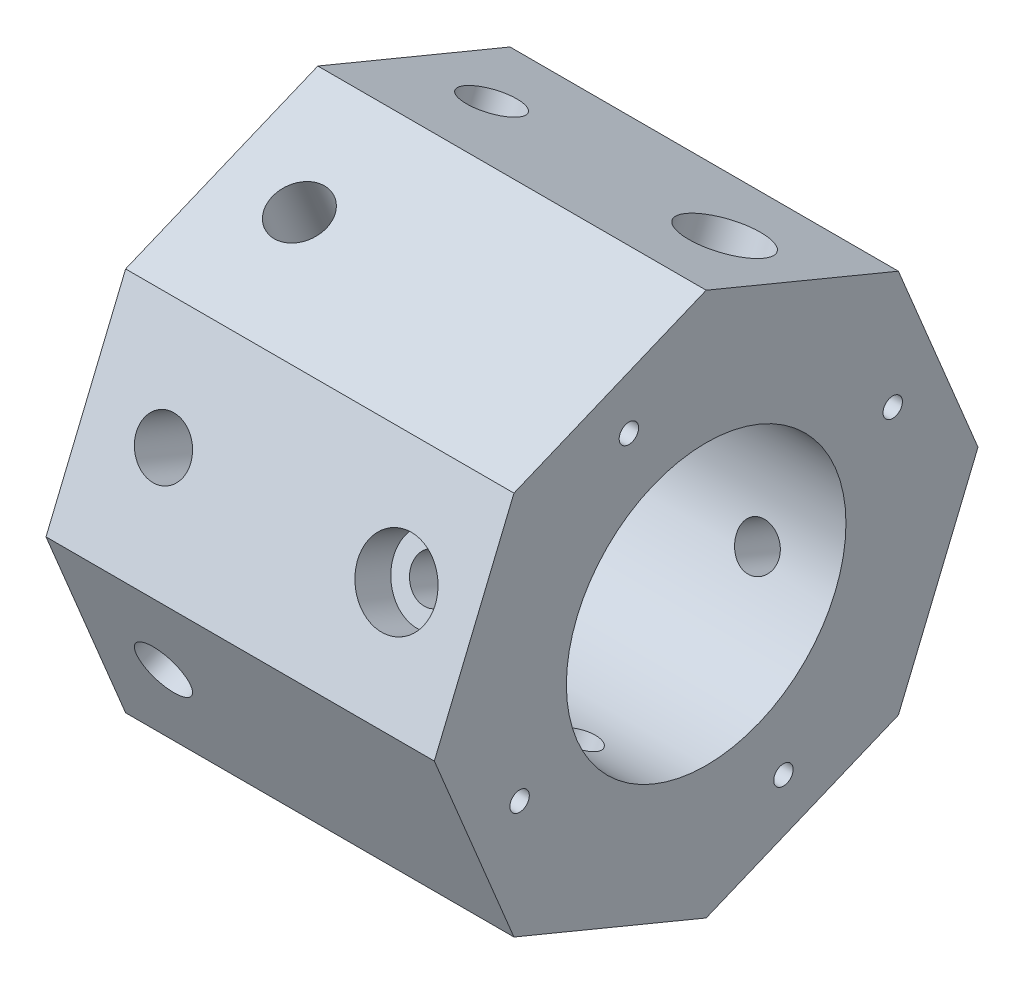
from build123d import *

# Parameters (mm, degrees)
SKETCH_1_R               = 18
EXTRUDE_1_DEPTH          = 25
SKETCH_2_R               = 5
CUT_EXTRUDE_1_DEPTH      = 5
SKETCH_4_R               = 2.75
CUT_EXTRUDE_2_DEPTH      = 23
PATTERN_CIRCULAR_1_COUNT = 8
PATTERN_CIRCULAR_2_COUNT = 4
PATTERN_CIRCULAR_3_COUNT = 4


with BuildPart() as part:
    # 草图1 → 凸台-拉伸1 (new, symmetric)
    with BuildSketch(Plane(origin=(0, 0, 0), x_dir=(0, 0, -1), z_dir=(1, 0, 0))):
        Polygon((24.748737342, 24.748737342), (0, 35), (-24.748737342, 24.748737342), (-35, 0), (-24.748737342, -24.748737342), (0, -35), (24.748737342, -24.748737342), (35, 0), align=None)
        Circle(SKETCH_1_R, mode=Mode.SUBTRACT)
    extrude(amount=EXTRUDE_1_DEPTH, both=True)

    # 草图2 → 切除-拉伸1 (cut)
    with BuildSketch(Plane(origin=(0, -29.874368671, 12.374368671), x_dir=(1, 0, 0), z_dir=(0, 0.9238795325112868, -0.3826834323650897))):
        with Locations(Location((15, 0, 0), (0, 0, 270))):
            Circle(SKETCH_2_R)
    cut_extrude_1 = extrude(amount=CUT_EXTRUDE_1_DEPTH, mode=Mode.SUBTRACT)

    # 草图4 → 切除-拉伸2 (cut)
    with BuildSketch(Plane(origin=(0, -25.254971008, 10.460951509), x_dir=(1, 0, 0), z_dir=(0, -0.9238795325112867, 0.38268343236508956))):
        with Locations(Location((15, 0, 0), (0, 0, 270))):
            Circle(SKETCH_4_R)
    cut_extrude_2 = extrude(amount=-CUT_EXTRUDE_2_DEPTH, mode=Mode.SUBTRACT)

    # 草图6 → M8x1.0 螺纹孔1 (revolve, cut)
    with BuildSketch(Plane(origin=(-15, -12.374368671, 29.874368671), x_dir=(0, -0.9238795325112867, -0.38268343236508995), z_dir=(1, 0, 0))):
        Polygon((0, 0), (0, 17.103012167), (3.5, 15), (3.5, 0), align=None)
    m8x1_0_1 = revolve(axis=Axis((-15, -14.804408466, 35.741003702), (0, 0.38268343236508995, -0.9238795325112867)), mode=Mode.SUBTRACT)

    # 阵列(圆周)1: M8x1.0 螺纹孔1 ×8 about axis
    pattern_circular_1_axis = Axis((25, 0, 0), (-1, 0, 0))
    for i in range(1, PATTERN_CIRCULAR_1_COUNT):
        add(m8x1_0_1.rotate(pattern_circular_1_axis, i * 360 / PATTERN_CIRCULAR_1_COUNT), mode=Mode.SUBTRACT)

    # 阵列(圆周)2: 切除-拉伸1, 切除-拉伸2 ×4 about axis
    pattern_circular_2_axis = Axis((0, 0, 0), (1, 0, 0))
    add([cut_extrude_1.rotate(pattern_circular_2_axis, i * 360 / PATTERN_CIRCULAR_2_COUNT) for i in range(1, PATTERN_CIRCULAR_2_COUNT)], mode=Mode.SUBTRACT)
    add([cut_extrude_2.rotate(pattern_circular_2_axis, i * 360 / PATTERN_CIRCULAR_2_COUNT) for i in range(1, PATTERN_CIRCULAR_2_COUNT)], mode=Mode.SUBTRACT)

    # 草图8 → M3x0.5 螺纹孔1 (revolve, cut)
    with BuildSketch(Plane(origin=(25, 9.949769241, -24.020867845), x_dir=(0, 0, -1), z_dir=(0, 1, 0))):
        Polygon((0, 0), (0, 8.251075774), (1.25, 7.5), (1.25, 0), align=None)
    m3x0_5_1 = revolve(axis=Axis((31.35, 9.949769241, -24.020867845), (-1, 0, 0)), mode=Mode.SUBTRACT)

    # 阵列(圆周)3: M3x0.5 螺纹孔1 ×4 about axis
    pattern_circular_3_axis = Axis((0, 0, 0), (1, 0, 0))
    for i in range(1, PATTERN_CIRCULAR_3_COUNT):
        add(m3x0_5_1.rotate(pattern_circular_3_axis, i * 360 / PATTERN_CIRCULAR_3_COUNT), mode=Mode.SUBTRACT)


solid = part.part
